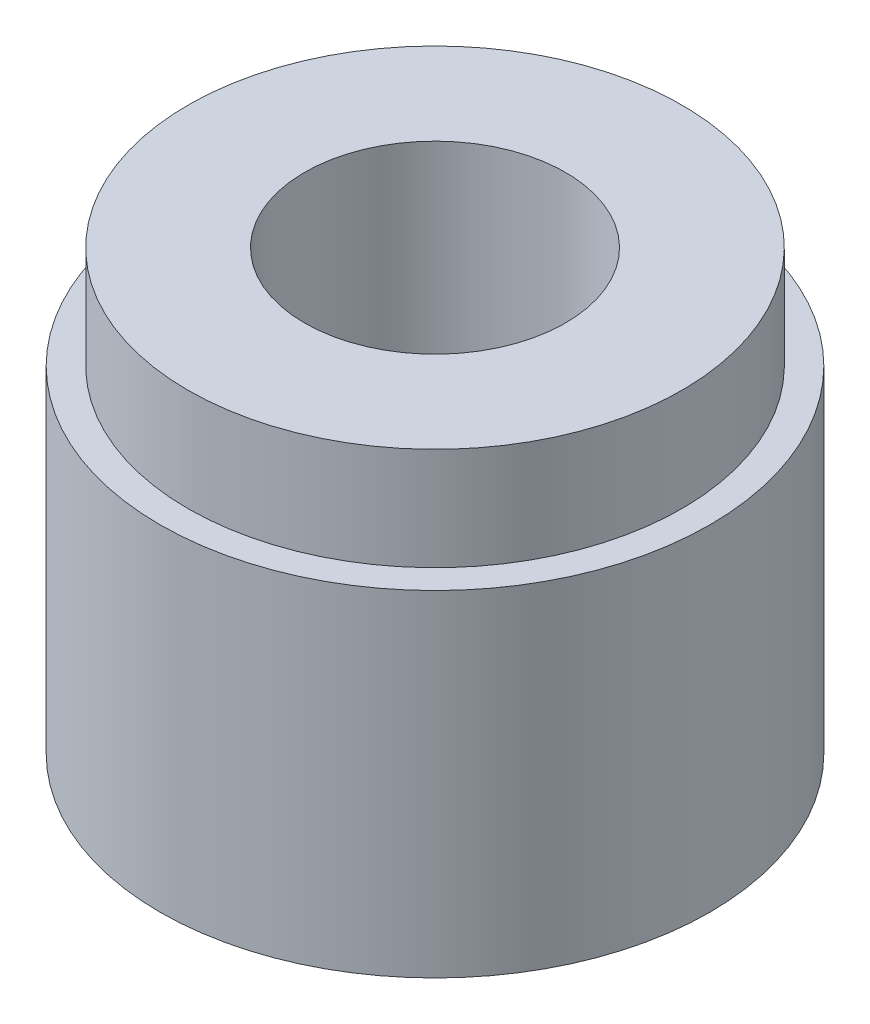
from build123d import *

# Parameters (mm, degrees)
SKETCH_1_R          = 59
SKETCH_1_R_2        = 28
EXTRUDE_1_DEPTH     = 94
SKETCH_2_OUTSIDE_W  = 158.306
SKETCH_2_OUTSIDE_H  = 158.306
SKETCH_2_OUTSIDE_R  = 53
CUT_EXTRUDE_1_DEPTH = 22


with BuildPart() as part:
    # 草图1 → 凸台-拉伸1 (new body)
    with BuildSketch(Plane(origin=(0, 0, 0), x_dir=(1, 0, 0), z_dir=(0, 1, 0))):
        with Locations(Location((0, 0, 0), (0, 0, 270))):
            Circle(SKETCH_1_R)
        with Locations(Location((0, 0, 0), (0, 0, 270))):
            Circle(SKETCH_1_R_2, mode=Mode.SUBTRACT)
    extrude(amount=EXTRUDE_1_DEPTH)

    # 草图2 outside → 切除-拉伸1 (cut)
    with BuildSketch(Plane(origin=(0, 94, 0), x_dir=(1, 0, 0), z_dir=(0, 1, 0))):
        Rectangle(SKETCH_2_OUTSIDE_W, SKETCH_2_OUTSIDE_H)
        with Locations(Location((0, 0, 0), (0, 0, 270))):
            Circle(SKETCH_2_OUTSIDE_R, mode=Mode.SUBTRACT)
    extrude(amount=-CUT_EXTRUDE_1_DEPTH, mode=Mode.SUBTRACT)


solid = part.part
